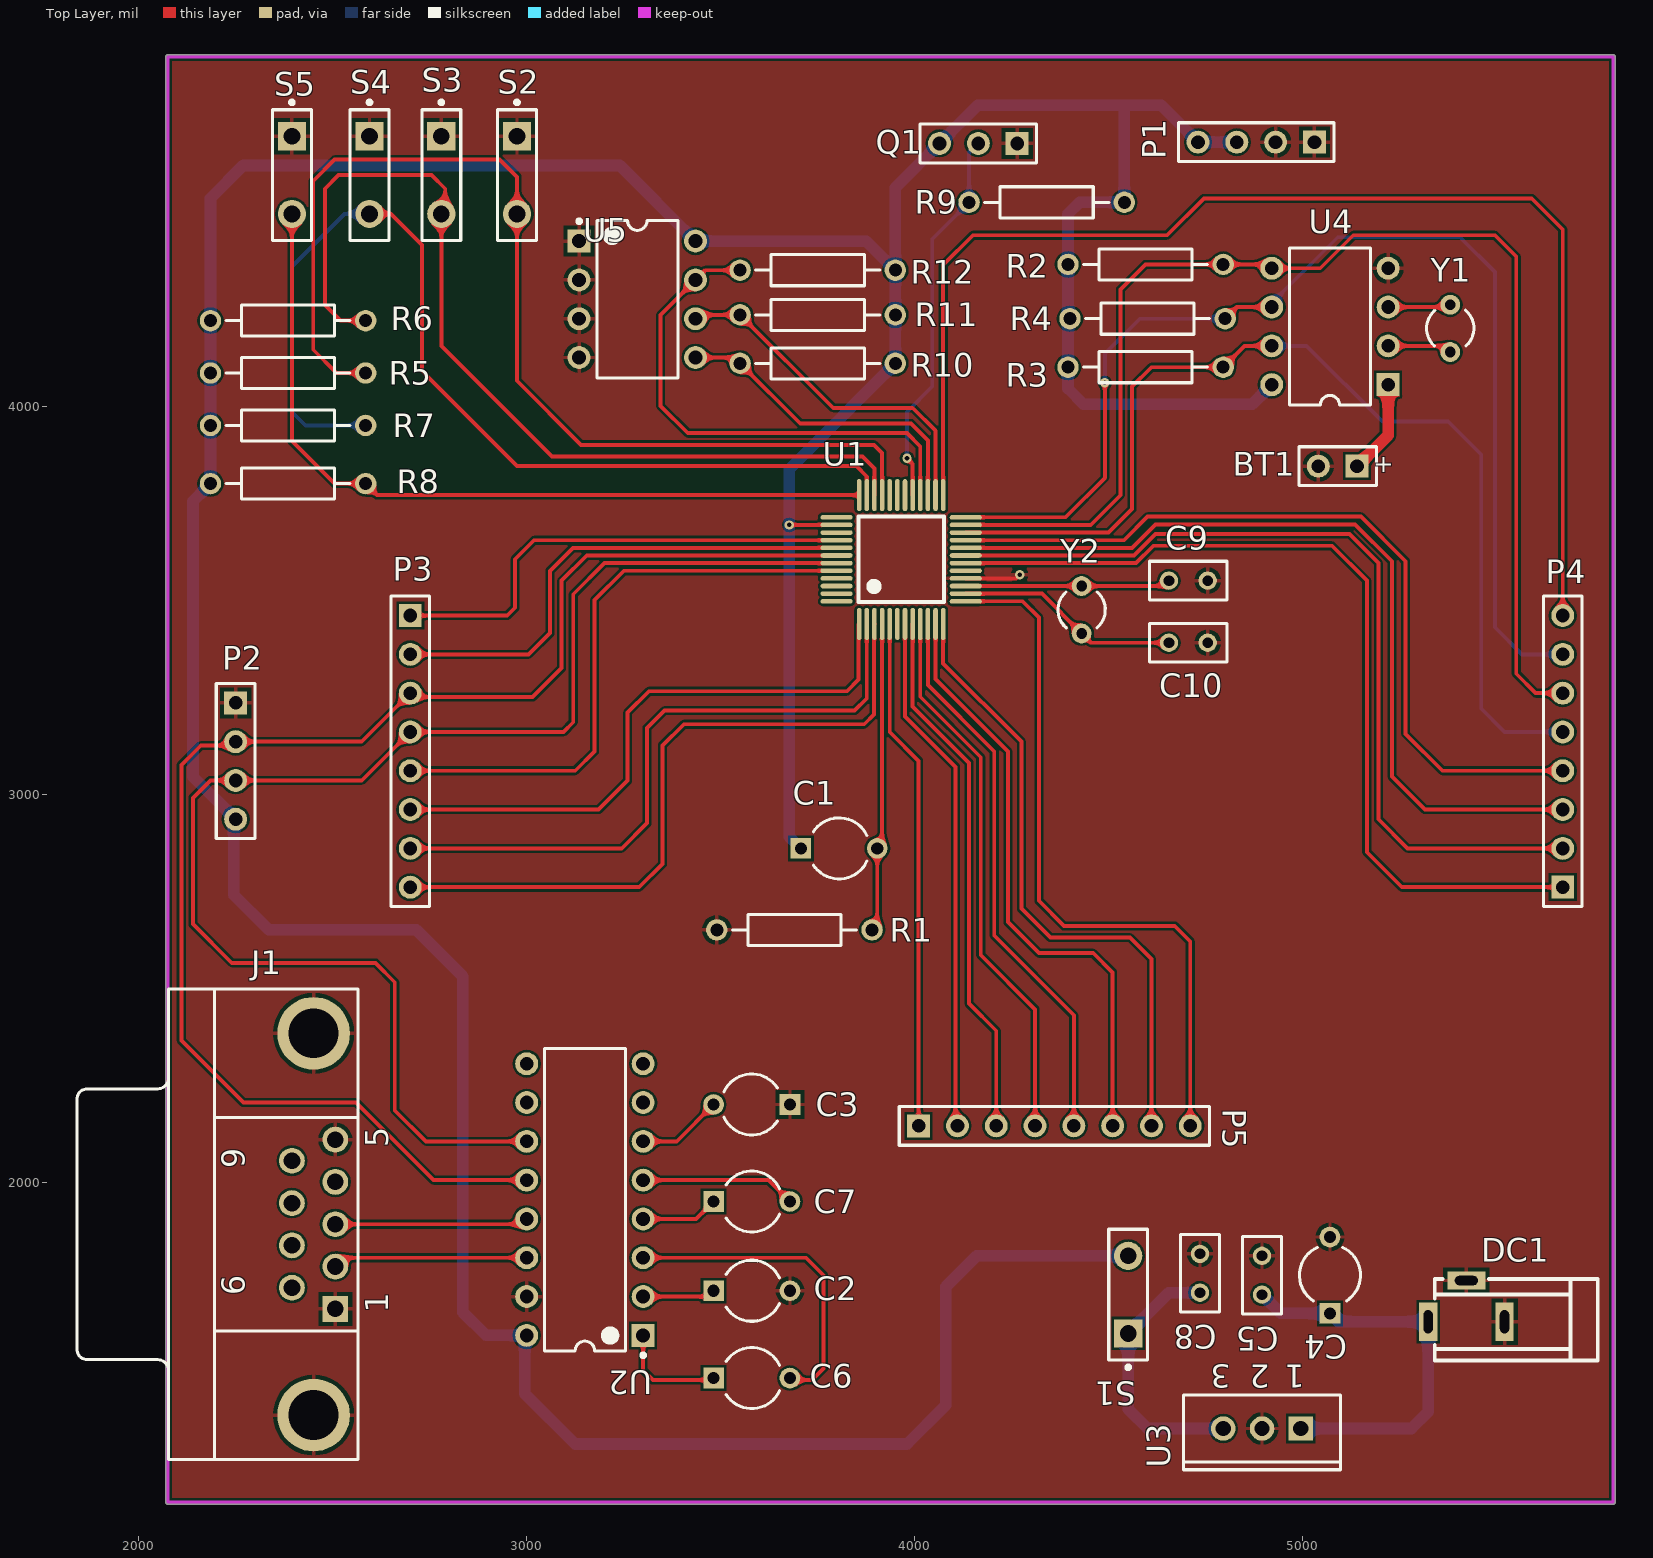
[diagram p0: Top Layer view]
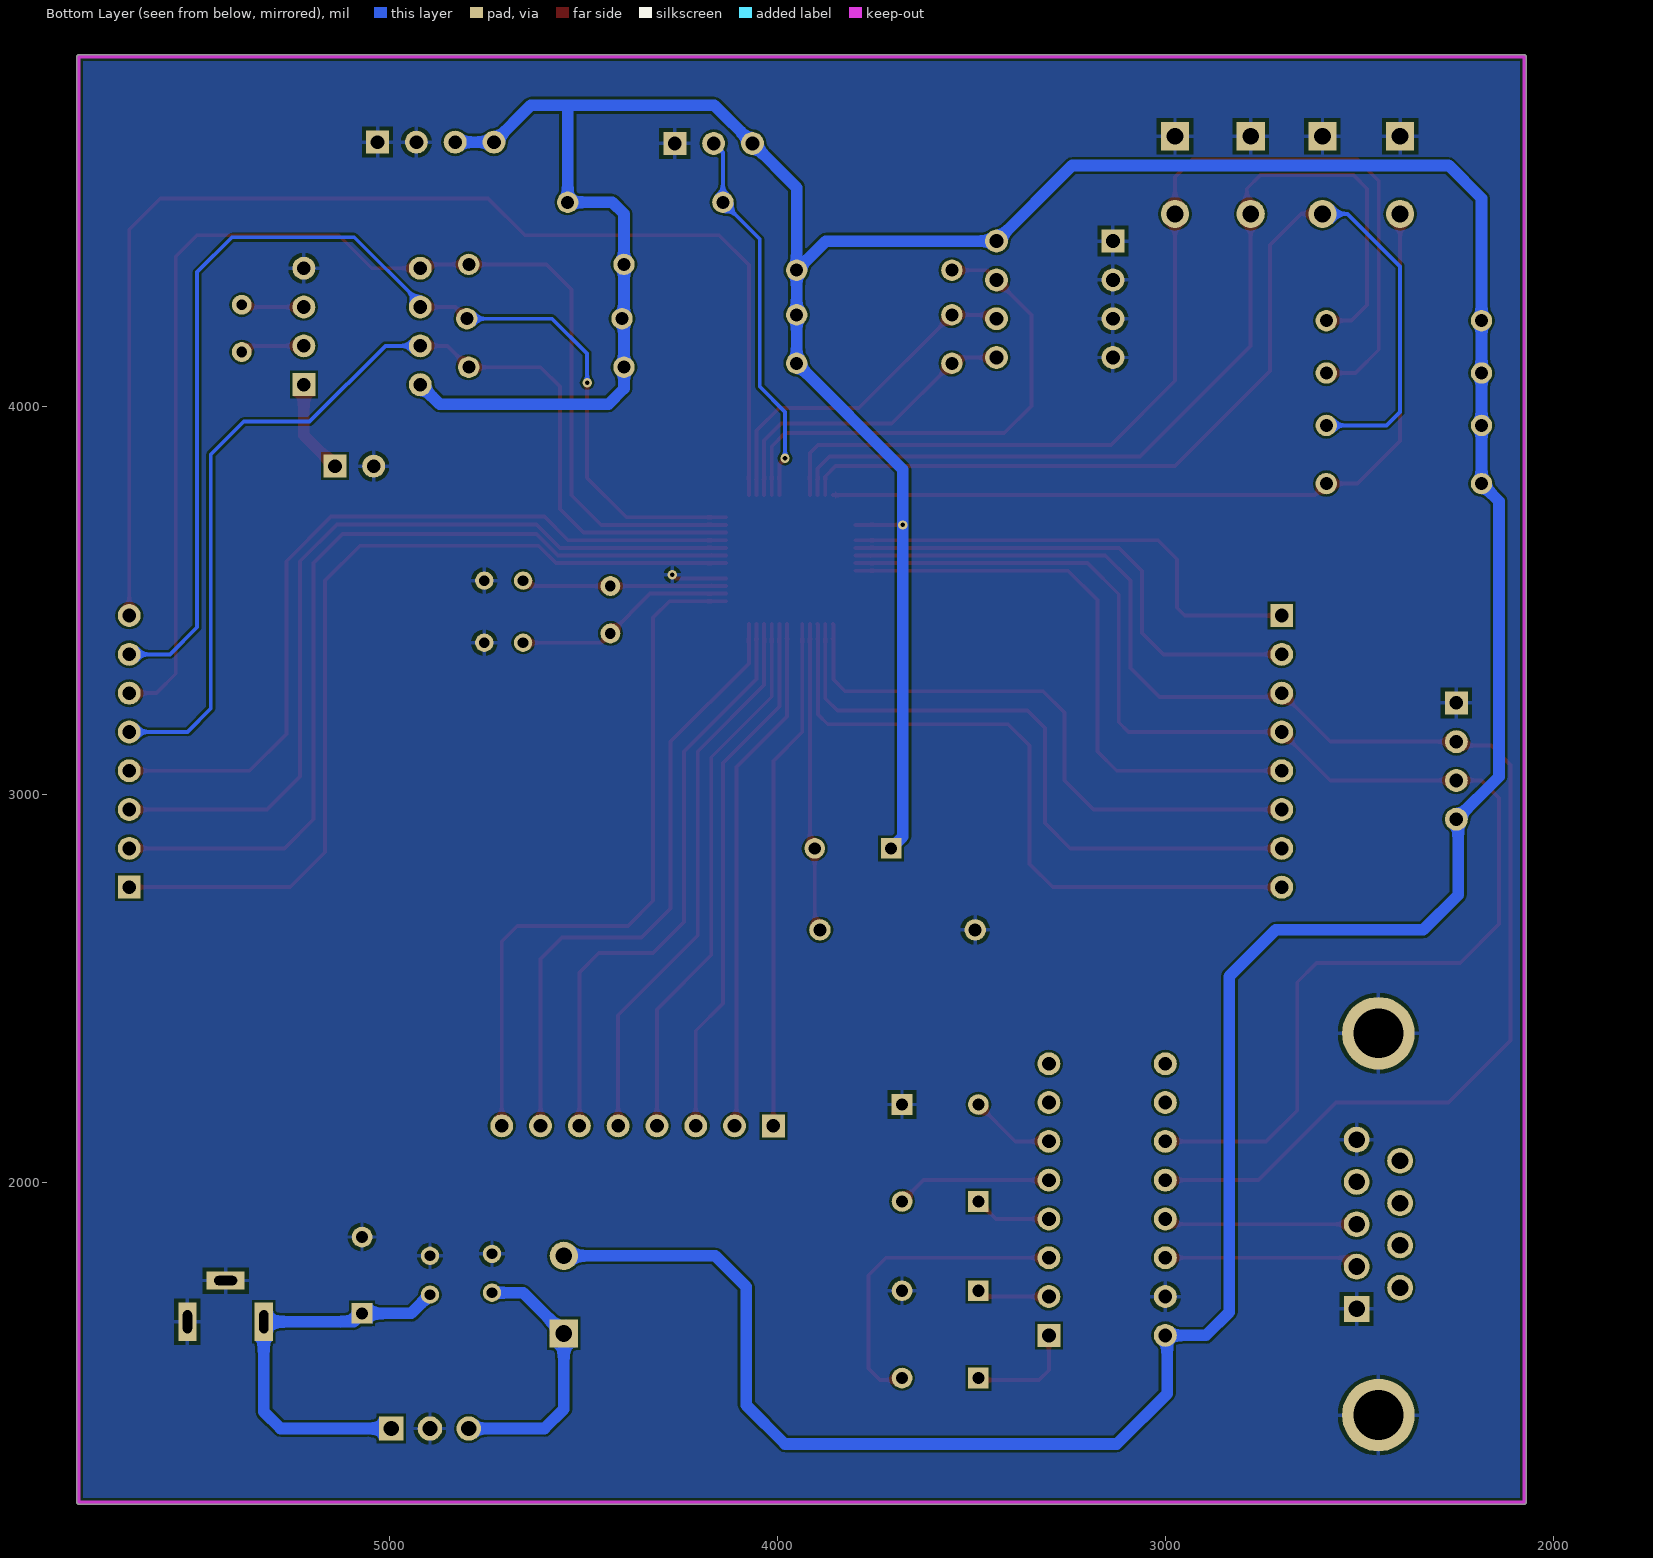
[diagram p1: Bottom Layer view, seen from below]
# Altium PCB MISC84364.PcbDoc
Units mil, origin at the board's own origin, x right, y up, seen from the top; angles counter-clockwise.
Board outline 3735.03 x 3735.03 mil, 2 copper layers (Top Layer, Bottom Layer); 43 components, 57 nets, 192 pads, 4 vias.

## Layer stack, top to bottom (the 12.6 mil dielectric is the usual default, probably not edited)
Top Solder: solder mask 0.4, Solder Resist, Dk 3.5
Top Layer: signal copper 1.4
Dielectric 1: dielectric 12.6, FR-4, Dk 4.8
Bottom Layer: signal copper 1.4
Bottom Solder: solder mask 0.4, Solder Resist, Dk 3.5

## Board outline
2069.99,1175 ccw(c2075,1175) 2075,1169.98 5800,1169.98 ccw(c5800,1175) 5805.02,1175 5805.02,4900 ccw(c5800,4900) 5800,4905.02 2075,4905.02 ccw(c2075,4900) 2069.99,4900

## Design rules (kind name [scope] priority, off if disabled: settings)
Clearance [All] p1: gap=6
HoleSize [All] p1: absolutevalues=TRUE maxlimit=99999 minlimit=1 maxpercent=80.000 minpercent=20.000
MinimumSolderMaskSliver [All] p1: minsoldermaskwidth=0
PolygonConnect [All] p1: connectstyle=Relief reliefconductorwidth=10 reliefentries=4 polygonreliefangle="90 Angle" airgapwidth=10
RoutingVias [All] p1: holewidth=28 width=50 viastyle="Through Hole" minholewidth=28 minwidth=50 maxholewidth=28 maxwidth=50
SilkToSilkClearance [All] p1: silktosilkclearance=0
SilkToSolderMaskClearance [IsPad] p1: minsilkscreentomaskgap=0 clearancetoexposedcopper=TRUE
SolderMaskExpansion [All] p1: expansion=4
Width [All] p1: maxlimit=30 minlimit=10 preferedwidth=10
26 further rules are at their usual default settings.

## Components (designator, comment, footprint, x,y, rotation, side; value= is the part's Value field where it differs from the comment)
BT1 "Battery" BAT-2 5090,3845 r180 top
C1 "Cap2" CAPR5-4X5 3805,2860 r0 top
C2 "Cap2" CAPR5-4X5 3580,1720 r0 top
C3 "Cap2" CAPR5-4X5 3580,2200 r180 top
C4 "Cap2" CAPR5-4X5 5070,1760 r90 top
C5 "Cap" RAD-0.1 4895,1760 r270 top
C6 "Cap2" CAPR5-4X5 3580,1495 r0 top
C7 "Cap2" CAPR5-4X5 3580,1950 r0 top
C8 "Cap" RAD-0.1 4735,1765 r270 top
C9 "Cap" RAD-0.1 4705,3550 r180 top
C10 "Cap" RAD-0.1 4705,3390 r180 top
DC1 "DC_Socket" DC-002 5323.15,1640 r0 top
J1 "D Connector 9" DSUB1.385-2H9 2076.89,1891.42 r90 top
P1 "Header 4" HDR1X4 5030,4680 r180 top
P2 "Header 4" HDR1X4 2250,3235 r270 top
P3 "Header 8" HDR1X8 2700,3460 r270 top
P4 "Header 8" HDR1X8 5670,2760 r90 top
P5 "Header 8" HDR1X8 4010,2145 r0 top
Q1 "DS18B20" HDR1X3 4263.94,4676.81 r180 top
R1 "Res2" AXIAL-0.4 3690,2650 r0 top
R2 "Res2" AXIAL-0.4 4595,4365 r180 top
R3 "Res2" AXIAL-0.4 4595,4100 r180 top
R4 "Res2" AXIAL-0.4 4600,4225 r0 top
R5 "Res2" AXIAL-0.4 2385,4085 r180 top
R6 "Res2" AXIAL-0.4 2385,4220 r180 top
R7 "Res2" AXIAL-0.4 2385,3950 r180 top
R8 "Res2" AXIAL-0.4 2385,3800 r180 top
R9 "Res2" AXIAL-0.4 4340,4525 r180 top
R10 "Res2" AXIAL-0.4 3750,4110 r180 top
R11 "Res2" AXIAL-0.4 3750,4235 r180 top
R12 "Res2" AXIAL-0.4 3750,4350 r180 top
S1 "SW-SPST" SPST-2 4550,1710 r90 top
S2 "SW-PB" SPST-2 2975,4595 r270 top
S3 "SW-PB" SPST-2 2780,4595 r270 top
S4 "SW-PB" SPST-2 2595,4595 r270 top
S5 "SW-PB" SPST-2 2395,4595 r270 top
U1 "STC32C5A60S2" "LQFP48 7X7" 3965,3605 r0 top
U2 "MAX232ACPE" PE16A 3150,1955 r180 top
U3 "MC7805BT" 221A-04 4895,1365 r180 top
U4 "DS1302" DIP8 5070,4205 r90 top
U5 "AT24C01" DIP-8 3285,4275 r0 top
Y1 "XTAL" R38 5380,4200 r180 top
Y2 "XTAL" R38 4430,3475 r0 top

## Footprints (in the part's own frame and the unit in brackets; to place one, negate y for a bottom-side part, rotate by r counter-clockwise, add the part's x,y. Pads: shape width x height; smd on the part's side, far side on the other; paste and mask are expansions set on the pad)
221A-04 [mm] "TO, Thru-Hole, Vertical, Heatsink Mounted; 3 In-Line Leads; Pitch 2.54 mm"
  rect 1.6x1.6 hole 1: 1(-2.54,0)
  round 1.6 hole 1: 2(0,0) 3(2.54,0)
  silkscreen extent -5.15,-2.2 5.15,2.7
AXIAL-0.4 [mm] "Axial Device, Thru-Hole; 2 Leads; 0.4 in Pin Spacing"
  round 1.4 hole 0.85: 1(-5.08,0) 2(5.08,0)
  silkscreen extent -4.06,-1.02 4.06,1.02
BAT-2 [mm] "Battery; 2 Leads"
  rect 1.5x1.5 hole 0.9: 1(-1.27,0)
  round 1.5 hole 0.9: 2(1.27,0)
  silkscreen extent -2.54,-1.27 2.54,1.27
CAPR5-4X5 [mm] "Capacitor; 2 Leads"
  rect 1.35x1.35 hole 0.8: 1(-2.5,0)
  round 1.35 hole 0.8: 2(2.5,0)
  silkscreen extent -1.69,-2 1.82,2
DC-002 [mm] "3.5X1.1mm"
  rect 1.2x2.5 hole 0.6 slot 1.5 at 90 deg: 1(0,0) 2(5,0)
  rect 2.5x1.2 hole 0.6 slot 1.5 at 0 deg: 3(2.5,2.7)
  silkscreen extent 0.43,-2.54 11.1,2.79, body extent -0.25,-2.55 11.05,2.8, height 7.3
DIP8 [mm] "DIP; 8 Leads; Row Spacing 7.62 mm; Pitch 2.54 mm"
  rect 1.5x1.5 hole 0.9: 1(-3.81,-3.81)
  round 1.5 hole 0.9: 2(-1.27,-3.81) 3(1.27,-3.81) 4(3.81,-3.81) 5(3.81,3.81) 6(1.27,3.81) 7(-1.27,3.81) 8(-3.81,3.81)
  silkscreen extent -5.15,-2.65 5.15,2.65
DIP-8 [mm] "DIP; 8 Leads; Row Spacing 7.62 mm; Pitch 2.54 mm"
  rect 1.5x1.5 hole 0.9: 1(-3.81,3.81)
  round 1.5 hole 0.9: 2(-3.81,1.27) 3(-3.81,-1.27) 4(-3.81,-3.81) 5(3.81,-3.81) 6(3.81,-1.27) 7(3.81,1.27) 8(3.81,3.81)
  silkscreen extent -3.93,-5.15 2.65,5.23, body extent -3.6,-5.15 3.6,5.15, height 5.08
DSUB1.385-2H9 [mm] "Connector; D Subminiature; 9 Position; Right Angle; Pitch 1.385 mm"
  rect 1.69x1.69 hole 1.09: 1(-5.54,-10.92)
  round 1.69 hole 1.09: 2(-2.77,-10.92) 3(0,-10.92) 4(2.77,-10.92) 5(5.54,-10.92) 6(-4.155,-8.08) 7(-1.385,-8.08) 8(1.385,-8.08) 9(4.155,-8.08)
  round 4.76 hole 3.26: 10(-12.495,-9.5) 11(12.495,-9.5)
  silkscreen extent -15.4,-12.4 15.4,6
HDR1X3 [mm] "Connector; Header; 3 Position"
  rect 1.5x1.5 hole 0.9: 1(0,0)
  round 1.5 hole 0.9: 2(2.54,0) 3(5.08,0)
  silkscreen extent -1.27,-1.27 6.35,1.27
HDR1X4 [mm] "Connector; Header; 4 Position"
  rect 1.5x1.5 hole 0.9: 1(0,0)
  round 1.5 hole 0.9: 2(2.54,0) 3(5.08,0) 4(7.62,0)
  silkscreen extent -1.27,-1.27 8.89,1.27
HDR1X8 [mm] "Connector; Header; 8 Position"
  rect 1.5x1.5 hole 0.9: 1(0,0)
  round 1.5 hole 0.9: 2(2.54,0) 3(5.08,0) 4(7.62,0) 5(10.16,0) 6(12.7,0) 7(15.24,0) 8(17.78,0)
  silkscreen extent -1.27,-1.27 19.05,1.27
"LQFP48 7X7" [mm]
  oval 0.3x2.1 smd: 1(-2.75,-4.227) 2(-2.25,-4.227) 3(-1.75,-4.227) 4(-1.25,-4.227) 5(-0.75,-4.227) 6(-0.25,-4.227) 7(0.25,-4.227) 8(0.75,-4.227) 9(1.25,-4.227) 10(1.75,-4.227) 11(2.25,-4.227) 12(2.75,-4.227) 25(2.75,4.202) 26(2.25,4.202) 27(1.75,4.202) 28(1.25,4.202) 29(0.75,4.202) 30(0.25,4.202) 31(-0.25,4.202) 32(-0.75,4.202) 33(-1.25,4.202) 34(-1.75,4.202) 35(-2.25,4.202) 36(-2.75,4.202)
  oval 2.1x0.3 smd: 13(4.227,-2.75) 14(4.227,-2.25) 15(4.227,-1.75) 16(4.227,-1.25) 17(4.227,-0.75) 18(4.227,-0.25) 19(4.227,0.25) 20(4.227,0.75) 21(4.227,1.25) 22(4.227,1.75) 23(4.227,2.25) 24(4.227,2.75) 37(-4.227,2.75) 38(-4.227,2.25) 39(-4.227,1.75) 40(-4.227,1.25) 41(-4.227,0.75) 42(-4.227,0.25) 43(-4.227,-0.25) 44(-4.227,-0.75) 45(-4.227,-1.25) 46(-4.227,-1.75) 47(-4.227,-2.25) 48(-4.227,-2.75)
  silkscreen extent -2.79,-2.79 2.79,2.79, body extent -4.51,-4.5 4.5,4.5, height 1.45
PE16A [mm] "DIP, 16-Leads, Row Spacing 7.62mm, Pitch 2.54mm, Body 19.18x6.99mm"
  rect 1.5x1.5 hole 0.9: 1(-3.81,8.89)
  round 1.5 hole 0.9: 2(-3.81,6.35) 3(-3.81,3.81) 4(-3.81,1.27) 5(-3.81,-1.27) 6(-3.81,-3.81) 7(-3.81,-6.35) 8(-3.81,-8.89) 9(3.81,-8.89) 10(3.81,-6.35) 11(3.81,-3.81) 12(3.81,-1.27) 13(3.81,1.27) 14(3.81,3.81) 15(3.81,6.35) 16(3.81,8.89)
  silkscreen extent -3.94,-9.9 2.65,10.31, body extent -3.3,-9.9 3.3,9.9, height 5.08
R38 [mm] "Crystal, Thru-Hole; 2 Leads; Body 3.1 x 8.2 mm (Dia.xH)"
  round 1.3 hole 0.7: 1(0,1.55) 2(0,-1.55)
  silkscreen extent -1.55,-1.19 1.55,1.17
RAD-0.1 [mm] "Radial Cap, Thru-Hole; 2 Leads; 0.1 in Pin Spacing"
  round 1.2 hole 0.7: 1(-1.27,0) 2(1.27,0)
  silkscreen extent -2.54,-1.27 2.54,1.27
SPST-2 [mm] "Switch; 2 Leads"
  rect 1.85x1.85 hole 1.1: 1(-2.54,0)
  round 1.85 hole 1.1: 2(2.54,0)
  silkscreen extent -4.89,-1.27 4.28,1.27

## Part data
BT1: "Multicell Battery"
C1 C2 C3 C4 C5 C6 C7 C8 C9 C10: "Capacitor"
J1: "Receptacle Assembly, 9 Position, Right Angle"
P1 P2: "Header, 4-Pin"
P3 P4 P5: "Header, 8-Pin"
Q1: "digital thermometer"
R1 R2 R3 R4 R5 R6 R7 R8 R9 R10 R11 R12: "Resistor"
S1: "Single-Pole, Single-Throw Switch"
S2 S3 S4 S5: "Switch"
U2: "+5V Powered, Multi-Channel RS-232 Driver/Receiver"
U3: "3-Terminal Positive Fixed Voltage Regulator"
U4: "Trickle Charge Timekeeping Chip"
U5: library part AT24C01BN-SP25-T, "1Kbit (128 x 8), 2-wire Bus Automotive Serial EEPROM with Write Protect, 2.5V, 8-Pin SOIC, Tape & Reel"
Y1 Y2: "Crystal Oscillator"

## Via types
v1: diameter 24, hole 12, Top Layer to Bottom Layer, 4 vias

## Nets (pads, with @x,y where several pads share a name; then routed paths per layer and width w, separated by ;. In a path a pad name is that pad's centre, name@x,y a point inside that pad or via, vN(x,y) a via of type N, cw(c..) or ccw(c..) an arc to the next point about the centre after c; other vN are vias at no path point)
GND: BT1.2 C2.2 C3.1 C4.2 C5.1 C8.1 C9.1 C10.1 DC1.2 DC1.3 J1.1 J1.5 J1.10 J1.11 P1.1 P1.2 P2.1 Q1.1 R1.1 S2.1 S3.1 S4.1 S5.1 U1.16 U2.15 U3.2 U4.4 U5.1 U5.2 U5.3 U5.4 | length 143
  Top Layer w10: U1.16 4260.79,3555.79 v1(4270.39,3565.39)
NetBT1_1: BT1.1 U4.1 | length 243.1
  Top Layer w30: BT1.1 5220,3925 U4.1
NetC2_1: C2.1 U2.2 | length 187.8
  Top Layer w10: U2.2 3466.57,1705 C2.1
NetC3_2: C3.2 U2.6 | length 220.9
  Top Layer w10: U2.6 3386.57,2105 C3.2
NetC4_1: C4.1 C5.2 DC1.1 U3.1 | length 1035
  Bottom Layer w30: C5.2 4943.43,1661.57 C4.1 5091.57,1640 DC1.1 5323.15,1408.15 5280,1365 U3.1
NetC6_1: C6.1 U2.1 | length 284
  Top Layer w10: U2.1 3300,1515 3325,1490 3476.57,1490 C6.1
NetC6_2: C6.2 U2.3 | length 824.7
  Top Layer w10: U2.3 3720,1805 3765,1760 3765,1520 3735,1490 3683.43,1490 C6.2
NetC7_1: C7.1 U2.4 | length 200.2
  Top Layer w10: U2.4 3436.57,1905 C7.1
NetC7_2: C7.2 U2.5 | length 401.2
  Top Layer w10: U2.5 3623.43,2005 C7.2
NetC8_2: C8.2 S1.1 U3.3 | length 689.2
  Bottom Layer w30: C8.2 4655,1715 S1.1 4550,1415 4600,1365 U3.3
NetJ1_2: J1.2 U2.14 | length 502.6
  Top Layer w10: J1.2 2529.45,1805 U2.14
NetJ1_3: J1.3 U2.13 | length 498.8
  Top Layer w10: J1.3 2986.42,1891.42 U2.13
NetU4_2: U4.2 Y1.1 | length 166.6
  Top Layer w10: U4.2 5363.98,4155 Y1.1
NetU4_3: U4.3 Y1.2 | length 162.5
  Top Layer w10: U4.3 5373.98,4255 Y1.2
P0_0: U1.37
P0_1: R8.1 S5.2 U1.36 | length 2104.5
  Top Layer w10: S5.2 2395,3910 2505,3800 R8.1 2614.58,3770.42 U1.36
P0_2: R7.1 S4.2 U1.35 | length 2635.6
  Top Layer w10: S4.2 2650,4495 2730,4415 2730,4090 2975,3845 3850,3845 3876.42,3818.58 U1.35
  Bottom Layer w10: R7.1 2430,3950 2395,3985 2395,4360 2530,4495 S4.2
P0_3: R6.1 S3.2 U1.34 | length 2485.2
  Top Layer w10: R6.1 2520,4220 2480,4260 2480,4560 2515,4595 2755,4595 2790,4560 2790,4505 S3.2 2780,4155 3065,3870 3865,3870 3896.1,3838.9 U1.34
P0_4: R5.1 S2.2 U1.33 | length 2812.8
  Top Layer w10: R5.1 2510,4085 2450,4145 2450,4580 2505,4635 2930,4635 2975,4590 S2.2 2975,4065 3140,3900 3895,3900 3915.79,3879.21 U1.33
P0_5: U1.32
P0_6: U1.31
P0_7: U1.30
P1_0: P3.1 U1.40 | length 1252.3
  Top Layer w10: P3.1 2950,3460 2970,3480 2970,3605 3019.21,3654.21 U1.40
P1_1: P3.2 U1.41 | length 1306
  Top Layer w10: P3.2 3005,3360 3060,3415 3060,3575 3119.53,3634.53 U1.41
P1_2: P2.2 P3.3 U1.42 U2.12 | length 3801.4
  Top Layer w10: U2.12 2760,2005 2560,2205 2270,2205 2110,2365 2110,3075 2160,3125 2240,3125 P2.2 2575,3135 P3.3 2710,3250 3015,3250 3090,3325 3090,3550 3154.84,3614.84 U1.42
P1_3: P2.3 P3.4 U1.43 U2.11 | length 3712.8
  Top Layer w10: U2.11 2740,2105 2660,2185 2660,2515 2610,2565 2240,2565 2140,2665 2140,2990 2185,3035 P2.3 2575,3035 P3.4 3095,3160 3120,3185 3120,3515 3200.16,3595.16 U1.43
P1_4: P3.5 U1.44 | length 1540.6
  Top Layer w10: P3.5 3125,3060 3175,3110 3175,3500 3250.47,3575.47 U1.44
P1_5: P3.6 U1.1 | length 1540.6
  Top Layer w10: P3.6 3185,2960 3260,3035 3260,3210 3315,3265 3825,3265 3855,3295 3855,3436.85 U1.1
P1_6: P3.7 U1.2 | length 1672.2
  Top Layer w10: P3.7 3245,2860 3310,2925 3310,3170 3355,3215 3845,3215 3876.42,3246.42 U1.2
P1_7: P3.8 U1.3 | length 1792
  Top Layer w10: P3.8 3290,2760 3350,2820 3350,3125 3405,3180 3870,3180 3895,3205 3895,3437.48 U1.3
P2_0: P4.1 U1.18 | length 2331.7
  Top Layer w10: U1.18 4570.16,3595.16 4615,3640 5075,3640 5165,3550 5165,2850 5255,2760 P4.1
P2_1: P4.2 U1.19 | length 2283.6
  Top Layer w10: U1.19 4564.84,3614.84 4620,3670 5120,3670 5195,3595 5195,2935 5270,2860 P4.2
P2_2: P4.3 U1.20 | length 2193.2
  Top Layer w10: U1.20 4559.53,3634.53 4620,3695 5135,3695 5230,3600 5230,3045 5315,2960 P4.3
P2_3: P4.4 U1.21 | length 2095.7
  Top Layer w10: U1.21 4539.21,3654.21 4600,3715 5150,3715 5265,3600 5265,3155 5360,3060 P4.4
P2_4: P4.5 R3.1 U1.22 U4.7 | length 2718.2
  Top Layer w10: U1.22 4498.9,3673.9 4560,3735 4560,4050 4610,4100 R3.1 4850,4155 U4.7
  Bottom Layer w10: U4.7 5010,4155 5205,3960 5375,3960 5460,3875 5460,3220 5520,3160 P4.5
P2_5: P4.6 R2.1 U1.23 U4.5 | length 3285
  Top Layer w10: U1.23 4453.58,3693.58 4530,3770 4530,4300 4595,4365 R2.1 4910,4365 U4.5 5045,4355 5130,4440 5495,4440 5550,4385 5550,3310 5600,3260 P4.6
P2_6: P4.7 R4.2 U1.24 U4.6 | length 3012.1
  Top Layer w10: U1.24 4388.27,3713.27 4490,3815 v1(4490,4060) ; R4.2 4830,4255 U4.6
  Bottom Layer w10: v1(4490,4060) 4490,4135 4580,4225 R4.2 ; U4.6 4920,4265 5090,4435 5405,4435 5495,4345 5495,3430 5565,3360 P4.7
P2_7: P4.8 U1.25 | length 3288.9
  Top Layer w10: U1.25 4073.27,4363.27 4150,4440 4650,4440 4745,4535 5590,4535 5670,4455 P4.8
P3_0: P5.1 U1.5 | length 1324.5
  Top Layer w10: U1.5 3935.47,3159.53 4010,3085 P5.1
P3_1: P5.2 U1.7 | length 1349.6
  Top Layer w10: U1.7 3974.84,3200.16 4105,3070 4105,2150 P5.2
P3_2: P5.3 U1.8 | length 1382.8
  Top Layer w10: U1.8 3994.53,3225.47 4140,3080 4140,2460 4210,2390 P5.3
P3_3: P5.4 U1.9 | length 1416.1
  Top Layer w10: U1.9 4014.21,3250.79 4170,3095 4170,2585 4310,2445 P5.4
P3_4: P5.5 U1.10 | length 1449.4
  Top Layer w10: U1.10 4033.9,3281.1 4205,3110 4205,2635 4410,2430 P5.5
P3_5: P5.6 U1.11 | length 1564.6
  Top Layer w10: U1.11 4053.58,3296.42 4240,3110 4240,2670 4320,2590 4460,2590 4510,2540 P5.6
P3_6: P5.7 U1.12 | length 1636
  Top Layer w10: U1.12 4073.27,3336.73 4275,3135 4275,2705 4350,2630 4555,2630 4610,2575 P5.7
P3_7: P5.8 U1.13 | length 1844.4
  Top Layer w10: U1.13 4278.27,3496.73 4320,3455 4320,2725 4385,2660 4670,2660 4710,2620 P5.8
P4_0: U1.17
P4_1: R12.2 U1.28 U5.7 | length 1325.4
  Top Layer w10: R12.2 3460,4350 U5.7 3345,4235 3345,4000 3415,3930 3980,3930 4014.21,3895.79 U1.28
P4_2: U1.39
P4_3: U1.6
P4_4: R11.2 U1.26 U5.6 | length 912.4
  Top Layer w10: U5.6 3445,4235 R11.2 3790,3995 3995,3995 4053.58,3936.42 U1.26
P4_5: R10.2 U1.27 U5.5 | length 828.2
  Top Layer w10: U5.5 3535,4125 R10.2 3705,3955 3990,3955 4033.9,3911.1 U1.27
P4_6: Q1.2 R9.2 U1.29 | length 995.7
  Top Layer w10: v1@3975,3870 v1(3980,3865) 3994.53,3850.47 U1.29
  Bottom Layer w10: v1(3980,3865) 3980,3985 4045,4050 4045,4430 R9.2 4140,4652.87 Q1.2
P4_7: C1.2 R1.2 U1.4 | length 799.3
  Top Layer w10: R1.2 3903.43,2663.43 C1.2 3915.79,2872.36 U1.4
VCC: C1.1 P1.3 P1.4 P2.4 Q1.3 R2.2 R3.2 R4.1 R5.2 R6.2 R7.2 R8.2 R9.1 R10.1 R11.1 R12.1 S1.2 U1.38 U2.16 U4.8 U5.8 | length 12027.5
  Top Layer w10: v1@3675,3695 v1(3676.42,3693.58) U1.38
  Bottom Layer w30: C1.1 3676.42,2890.16 v1(3676.42,3693.58) 3676.42,3836.42 R10.1 R11.1 R12.1 ; S1.2 4160,1810 4080,1730 4080,1425 3980,1325 3125,1325 2995,1455 2995,1600 U2.16 2895,1605 2835,1665 2835,2530 2715,2650 2335,2650 2245,2740 2245,2930 P2.4 2140,3045 2140,3755 R8.2 R7.2 R5.2 R6.2 2185,4535 2270,4620 3240,4620 U5.8 3875,4425 R12.1 ; P1.3 P1.4 4635,4775 4535,4775 ; U4.8 4870,4005 4435,4005 4395,4045 R3.2 R2.2 4395,4495 4425,4525 R9.1 4540,4770 4535,4775 ; R12.1 3950,4562.87 Q1.3 4162.13,4775 4535,4775
XTAL1: C9.2 U1.15 Y2.1 | length 529.4
  Top Layer w10: U1.15 4429.92,3536.1 Y2.1 4641.02,3536.02 C9.2
XTAL2: C10.2 U1.14 Y2.2 | length 575.9
  Top Layer w10: U1.14 4327.56,3516.42 Y2.2 4453.98,3390 C10.2
pads on no net: J1.4 J1.6 J1.7 J1.8 J1.9 U1.45 U1.46 U1.47 U1.48 U2.7 U2.8 U2.9 U2.10

## Polygon pours and split planes (outlines as drawn)
GND on Bottom Layer "D" (solid, remove dead copper, pour order 2): 1605,5355 6675,5355 6705,5325 6475,5095 6475,400 2145,400 1585,960
GND on Top Layer "D" (solid, remove dead copper, pour order 0): 1580,5105 1595,5120 6545,5120 6545,1275 6215,945 5965,695 1190,695

## Keep-outs
Keep-Out Layer:
  lines w10: 2075,2485 2075,4900 5800,4900 5800,1175 2075,1175 2075,2715